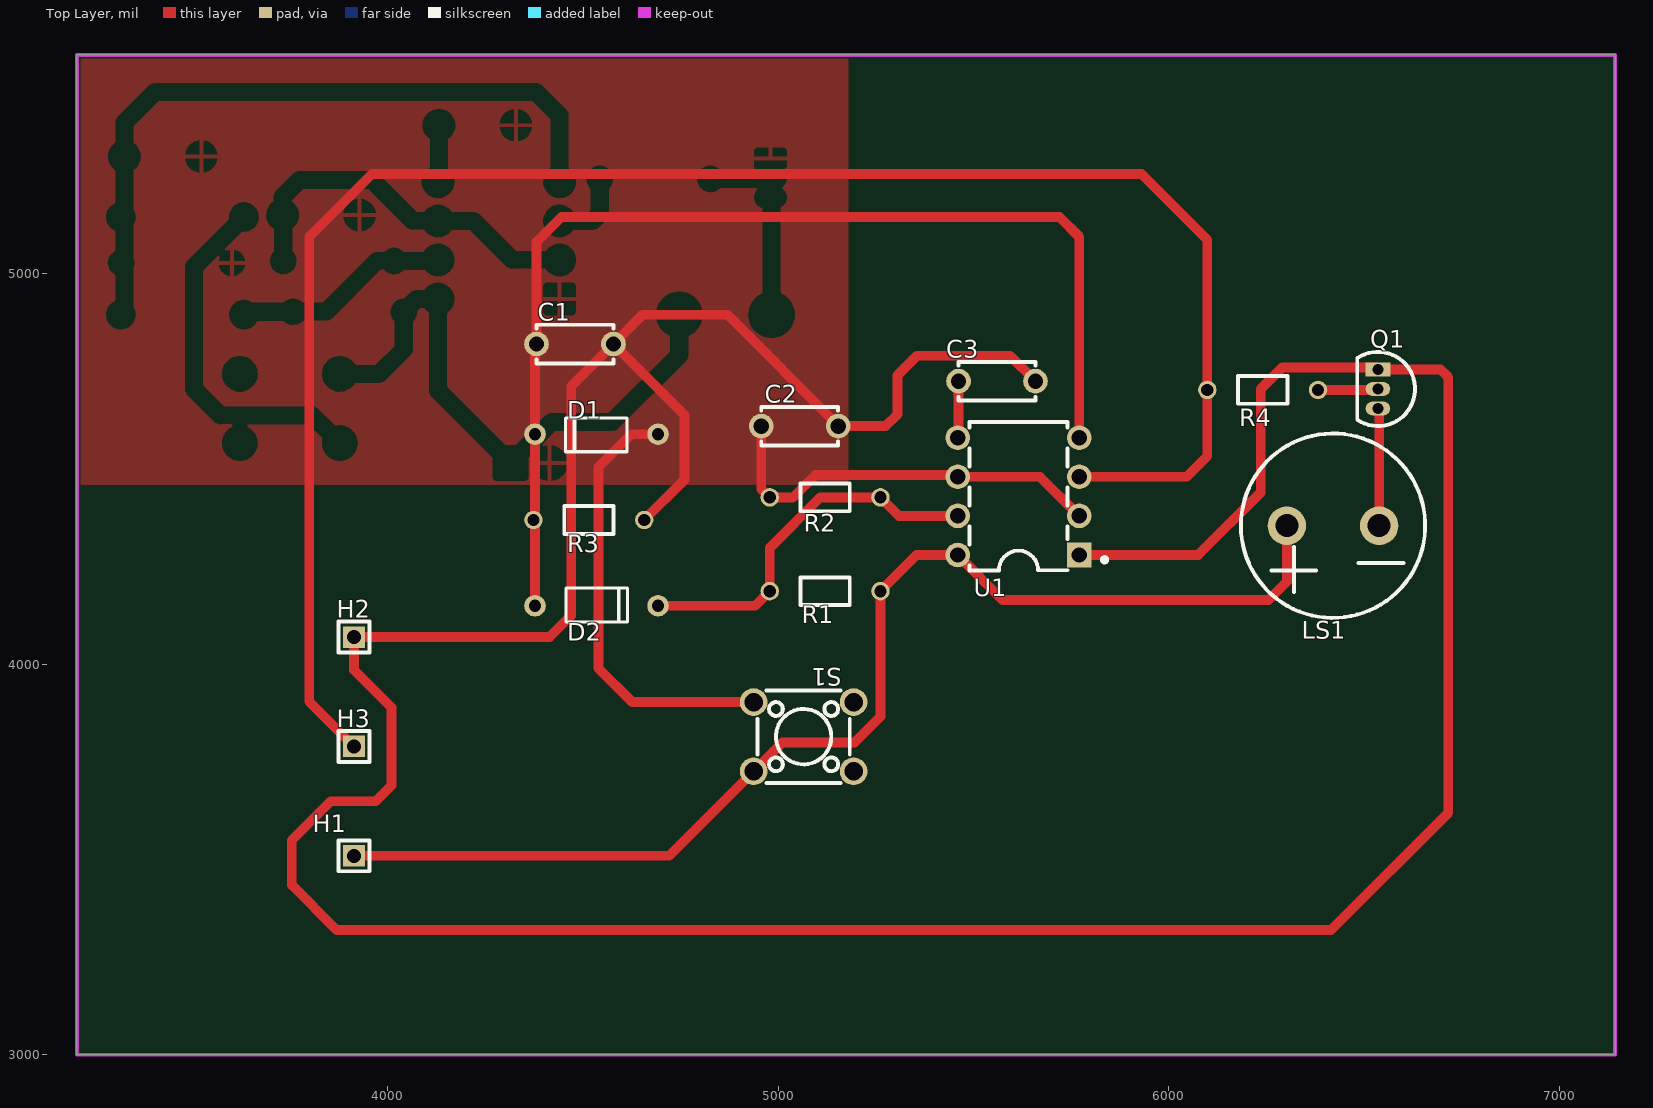
[diagram p0: Top Layer view]
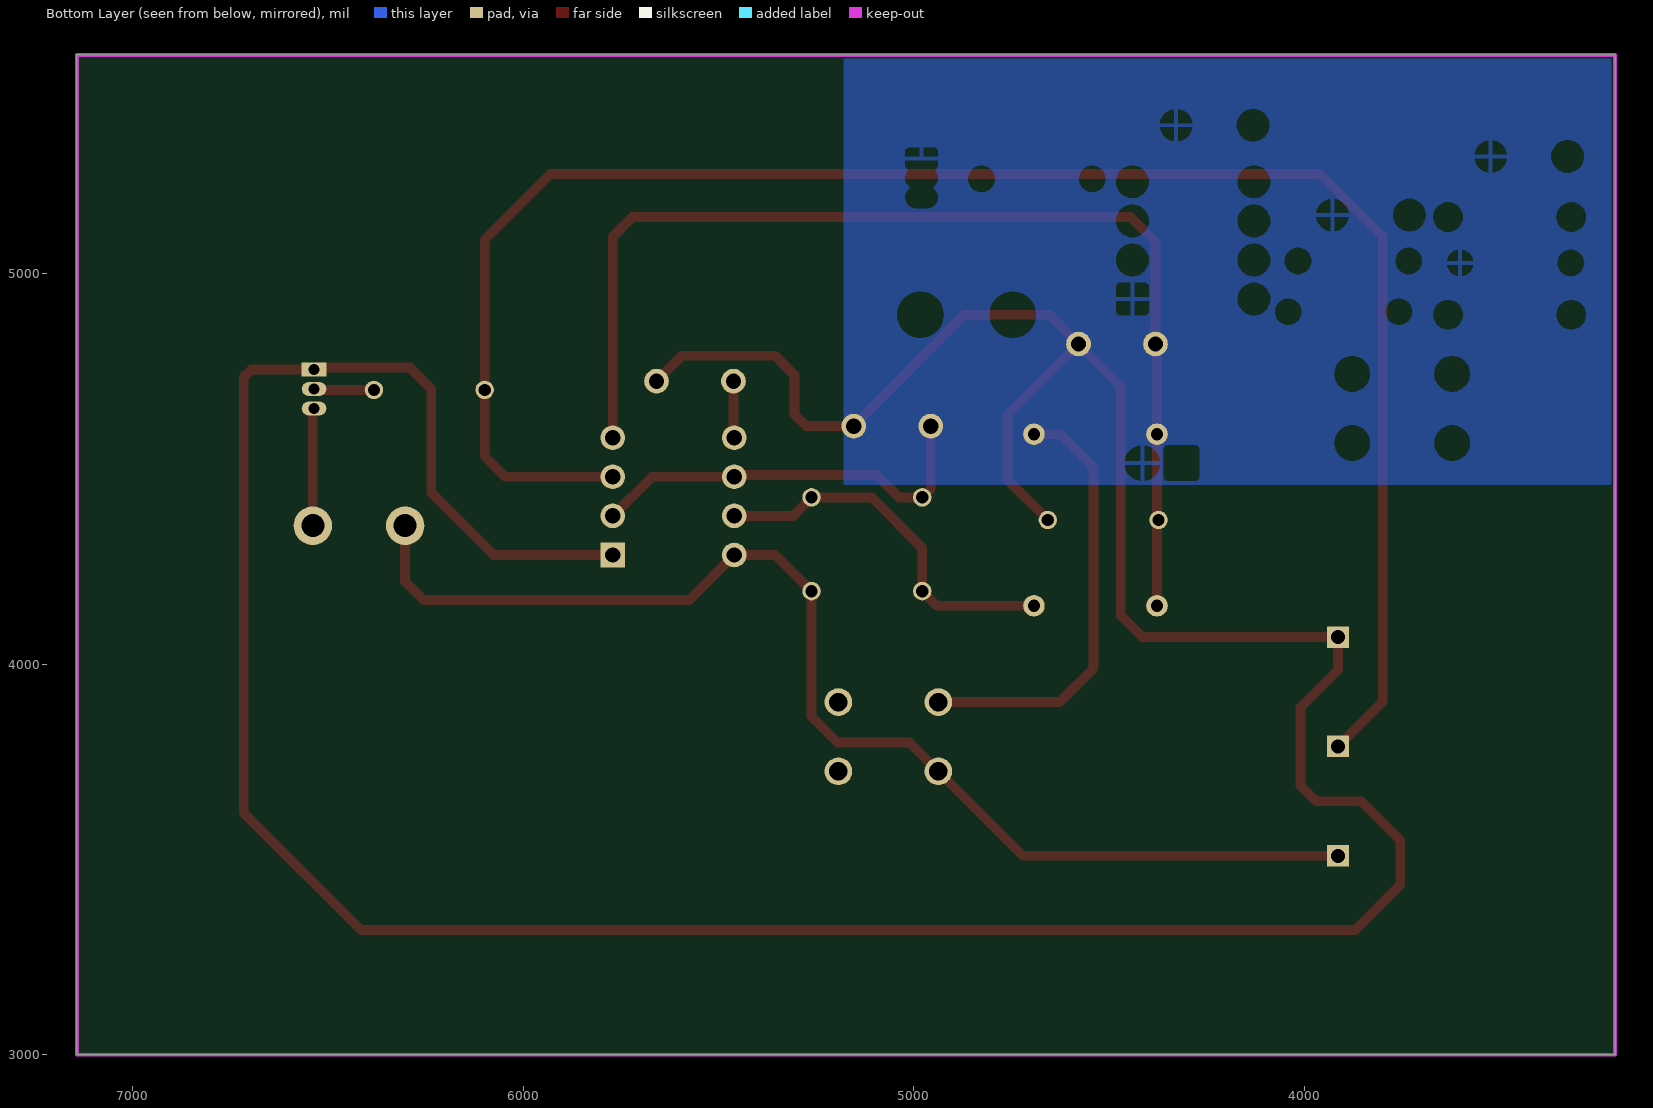
[diagram p1: Bottom Layer view, seen from below]
# Altium PCB MISC52004.pcbdoc
Units mil, origin at the board's own origin, x right, y up, seen from the top; angles counter-clockwise.
Board outline 3937.01 x 2559.06 mil, 2 copper layers (Top Layer, Bottom Layer), stack 62.206 mil thick; 16 components, 10 nets, 38 pads, 0 vias.

## Layer stack, top to bottom
Top Solder Mask Layer: solder mask 0.394, Dk 3.3
Top Layer: signal copper 1.379
Dielectric1: surface 59.449, FR4, Dk 4.5
Bottom Layer: signal copper 1.378
Bottom Solder Mask Layer: solder mask 0.394, Dk 3.3

## Board outline
3205,5559.06 3205,3000 7142.01,3000 7142.01,5559.06

## Design rules (kind name [scope] priority, off if disabled: settings)
BoardOutlineClearance copperThickness2oz_1 [All] p2 off: genericclearance=7.99 ignorepadtopadclearanceinfootprint=FALSE except(0: Arc-SplitContinuation Track-SplitContinuation SMDPad-SplitContinuation THPad-SplitContinuation Via-SplitContinuation Fill-SplitContinuation Region-SplitContinuation Poly-SplitContinuation Text-SplitContinuation Hole-SplitContinuation; 5.98: Arc-CutoutEdge SMDPad-CutoutEdge THPad-CutoutEdge Via-CutoutEdge Fill-CutoutEdge Region-CutoutEdge Text-CutoutEdge; 6.93: Hole-OutlineEdge Hole-CutoutEdge; 10: Poly-OutlineEdge Poly-CutoutEdge; 11.81: Arc-OutlineEdge Track-OutlineEdge SMDPad-OutlineEdge THPad-OutlineEdge Via-OutlineEdge Fill-OutlineEdge Region-OutlineEdge Text-OutlineEdge Track-CutoutEdge)
BoardOutlineClearance copperThickness1oz_1 [All] p4: genericclearance=4.02 ignorepadtopadclearanceinfootprint=FALSE except(0: Arc-SplitContinuation Track-SplitContinuation SMDPad-SplitContinuation THPad-SplitContinuation Via-SplitContinuation Fill-SplitContinuation Region-SplitContinuation Poly-SplitContinuation Text-SplitContinuation Hole-SplitContinuation; 6: SMDPad-CutoutEdge THPad-CutoutEdge Via-CutoutEdge Fill-CutoutEdge Region-CutoutEdge Text-CutoutEdge; 6.93: Hole-OutlineEdge Hole-CutoutEdge; 10: Poly-OutlineEdge Poly-CutoutEdge; 11.8: Arc-OutlineEdge Track-OutlineEdge SMDPad-OutlineEdge THPad-OutlineEdge Via-OutlineEdge Fill-OutlineEdge Region-OutlineEdge Text-OutlineEdge; 11.81: Arc-CutoutEdge Track-CutoutEdge)
Clearance copperThickness2oz [All] p1 off: gap=7.99 ignorepadtopadclearanceinfootprint=FALSE except(5.98: SMDPad-Track SMDPad-SMDPad THPad-Track SMDPad-THPad THPad-THPad Track-Via SMDPad-Via THPad-Via Via-Via Fill-Track Region-Track Fill-SMDPad Region-SMDPad Fill-THPad Region-THPad Fill-Via Region-Via Fill-Fill Fill-Region Region-Region Arc-Track Arc-SMDPad Arc-THPad Arc-Via Fill-Arc Region-Arc Arc-Arc Text-Track SMDPad-Text Text-THPad Text-Via Fill-Text Region-Text Arc-Text Text-Text; 6.93: Hole-Track Hole-SMDPad Hole-THPad Hole-Via Fill-Hole Region-Hole Hole-Arc Hole-Text; 10: Poly-Track Poly-SMDPad Poly-THPad Poly-Via Poly-Fill Poly-Region Poly-Poly Poly-Arc Poly-Text Poly-Hole)
Clearance copperThickness1oz [All] p3: gap=4.02 ignorepadtopadclearanceinfootprint=FALSE except(5.98: SMDPad-Track SMDPad-SMDPad THPad-Track SMDPad-THPad THPad-THPad Track-Via SMDPad-Via THPad-Via Via-Via Fill-Track Region-Track Fill-SMDPad Region-SMDPad Fill-THPad Region-THPad Fill-Via Region-Via Fill-Fill Fill-Region Region-Region; 6: Arc-Track Arc-SMDPad Arc-THPad Arc-Via Fill-Arc Region-Arc Arc-Arc Text-Track SMDPad-Text Text-THPad Text-Via Fill-Text Region-Text Arc-Text Text-Text; 6.93: Hole-Track Hole-SMDPad Hole-THPad Hole-Via Fill-Hole Region-Hole Hole-Arc Hole-Text; 10: Poly-Track Poly-SMDPad Poly-THPad Poly-Via Poly-Fill Poly-Region Poly-Poly Poly-Arc Poly-Text Poly-Hole)
Creepage creepage [All] p1: checkdistance=0 ignoreinternallayers=TRUE applytopolygonpour=TRUE
DiffPairsRouting differentialPair [All] p1: maxlimit=6 minlimit=6 mostfreqgap=6 toplayer_minwidth=5 toplayer_prefwidth=10 toplayer_maxwidth=100 toplayer_mingap=6 toplayer_prefgap=6 toplayer_maxgap=6 bottomlayer_minwidth=5 bottomlayer_prefwidth=10 bottomlayer_maxwidth=100 bottomlayer_mingap=6 bottomlayer_prefgap=6 bottomlayer_maxgap=6 maxuncoupledlength=10
HoleToHoleClearance otherClearance [All] p1: gap=11.81 allowstackedmicrovias=TRUE
Length netLength [All] p1: minlimit=0 maxlimit=0
MatchedLengths netLengthTolerance [All] p1: tolerance=1000
PasteMaskExpansion pasteMaskExpansion [All] p1: expansion=0
PlaneConnect innerPlane [All] p1: planeconnectstyle=Relief reliefexpansion=20 reliefentries=4 reliefconductorwidth=10 reliefairgap=10
PolygonConnect copperRegion [(InNet('GND'))] p1: connectstyle=Relief reliefconductorwidth=10 reliefentries=4 polygonreliefangle="90 Angle" airgapwidth=10 via.connectstyle=Relief via.reliefconductorwidth=10 via.reliefentries=4 via.polygonreliefangle="90 Angle" via.airgapwidth=10
RoutingVias viaSize [All] p1: holewidth=12.01 width=24.02 viastyle="Through Hole" minholewidth=11.81 minwidth=19.68 maxholewidth=248.03 maxwidth=393.7
SolderMaskExpansion solderMaskExpansion [IsVia] p1: expansion=-1000 istentingtop=TRUE
SolderMaskExpansion solderMaskExpansion [All] p2: expansion=2 istentingtop=FALSE
Width copperThickness2oz_2 [All] p1 off: maxlimit=100 minlimit=8 preferedwidth=10
Width copperThickness1oz_2 [All] p2: maxlimit=100 minlimit=5 preferedwidth=10

## Components (designator, comment, footprint, x,y, rotation, side; value= is the part's Value field where it differs from the comment)
C1 "100nF" CAP-TH_L5.0-W2.5-P5.00-D1.0 4479.88,4819.06 r0 top
C2 "0.1uF" CAP-TH_L5.0-W2.5-P5.00-D1.0 5055,4609.06 r0 top
C3 "0.01uF" CAP-TH_L5.0-W2.5-P5.00-D1.0 5560,4724.06 r0 top
D1 "1N4148" DO-35_BD2.2-L4.0-D0.50_1N4148 4535,4588.25 r180 top
D2 "1N4148" DO-35_BD2.2-L4.0-D0.50_1N4148 4535,4149.06 r0 top
H1 "" HDR-TH_1P-V-M_XKB_X4611WV-01I-C28D40 3914.27,3509.06 r0 top
H2 "" HDR-TH_1P-V-M_XKB_X4611WV-01I-C28D40 3914.27,4069.06 r0 top
H3 "" HDR-TH_1P-V-M_XKB_X4611WV-01I-C28D40 3914.27,3789.06 r0 top
LS1 "buzzer" BUZ-TH_BD12.0-P6.00-D0.9-RD 6420,4354.06 r180 top
Q1 "" S8050_TO_92 6535,4704.06 r270 top
R1 "10kΩ" Res_1/8W 5120,4184.06 r0 top
R2 "5kΩ" Res_1/8W 5120,4424.06 r0 top
R3 "10kΩ" Res_1/8W 4515.26,4371.13 r180 top
R4 "120Ω" Res_1/8W 6240,4699.06 r0 top
S1 "" SW-TH_4P-L6.0-W6.0-P4.50-LS6.5 5065,3814.06 r0 top
U1 "LM555CM" PDIP-8_L9.6-W6.4-P2.54-LS7.9-BL-1 5615,4429.06 r90 top

## Footprints (in the part's own frame and the unit in brackets; to place one, negate y for a bottom-side part, rotate by r counter-clockwise, add the part's x,y. Pads: shape width x height; smd on the part's side, far side on the other; paste and mask are expansions set on the pad)
BUZ-TH_BD12.0-P6.00-D0.9-RD [mm]
  round 2.5 hole 1.5 paste+0 mask+0.05: 1(-3,0) 2(3,0)
  silkscreen extent -5.99,-5.99 5.99,5.99
CAP-TH_L5.0-W2.5-P5.00-D1.0 [mm]
  round 1.6 hole 1: 1(-2.5,0) 2(2.5,0)
  silkscreen extent -2.5,-1.27 2.5,1.25
DO-35_BD2.2-L4.0-D0.50_1N4148 [mm]
  round 1.4 hole 0.8 paste+0 mask+0.05: 1(-4,0) 2(4,0)
  silkscreen extent -1.98,-1.06 2.02,1.14
HDR-TH_1P-V-M_XKB_X4611WV-01I-C28D40 [mm]
  rect 1.4x1.4 hole 0.9: 1(0,0)
  silkscreen extent -1,-1 1,1
PDIP-8_L9.6-W6.4-P2.54-LS7.9-BL-1 [mil]
  rect 63x63 hole 39.37: 1(-150,-155.51)
  round 63 hole 39.37: 2(-50,-155.51) 3(50,-155.51) 4(150,-155.51) 5(150,155.52) 6(50,155.52) 7(-50,155.52) 8(-150,155.52)
  silkscreen extent -190,-226 190,125
Res_1/8W [mil]
  round 47.2 hole 31.5 paste+0 mask+2: 1(-141.7,2.48) 2(141.7,2.48)
  silkscreen extent -63,-33 63,38
S8050_TO_92 [mil]
  rect 35.4x63 hole 27.6 paste+0 mask+2: 1(-50,0)
  oval 35.4x63 hole 27.6 paste+0 mask+2: 2(0,0) 3(50,0)
  silkscreen extent -95,-53 95,95
SW-TH_4P-L6.0-W6.0-P4.50-LS6.5 [mm]
  round 1.8 hole 1.2: 1(-3.25,2.25) 2(3.25,2.25) 3(-3.25,-2.25) 4(3.25,-2.25)
  silkscreen extent -3,-3 3,3

## Nets (pads, with @x,y where several pads share a name; then routed paths per layer and width w, separated by ;. In a path a pad name is that pad's centre, name@x,y a point inside that pad or via, vN(x,y) a via of type N, cw(c..) or ccw(c..) an arc to the next point about the centre after c; other vN are vias at no path point)
$1N2: D1.1 S1.1 | length 1135.2
  Top Layer w25: D1.1 4624.19,4588.25 4540,4504.06 4540,3989.06 4626.42,3902.64 S1.1
$1N3: C1.1 D1.2 D2.1 R3.2 U1.4 | length 2883.9
  Top Layer w25: D2.1 D1.2 4377.52,4815.12 C1.1 4381.46,5080.51 4445,5144.06 5720,5144.06 5770.51,5093.55 U1.4
$1N4: D2.2 R1.1 R2.2 U1.7 | length 966.5
  Top Layer w25: D2.2 4940.82,4149.06 R1.1 4978.3,4297.36 5107.48,4426.53 R2.2 5309.18,4379.06 U1.7
$1N7: C2.1 R2.1 U1.2 U1.6 | length 1051.1
  Top Layer w25: C2.1 4956.57,4448.26 R2.1 5037.48,4426.53 5095,4484.06 5454.49,4484.06 U1.6 5670.51,4479.06 U1.2
$1N9: C3.1 U1.5 | length 145.9
  Top Layer w25: U1.5 5461.57,4581.14 C3.1
$1N10: H3.1 R4.1 U1.3 | length 4689.9
  Top Layer w25: H3.1 3800,3903.33 3800,5094.06 3960,5254.06 5930,5254.06 6098.3,5085.76 R4.1 6098.3,4532.36 6045,4479.06 U1.3
$1N11: Q1.2 R4.2 | length 154.3
  Top Layer w25: R4.2 6532.48,4701.53 Q1.2
$1N12: LS1.1 Q1.3 | length 301.3
  Top Layer w25: Q1.3 6538.11,4650.95 LS1.1
GND: C1.2 C2.2 C3.2 H2.1 Q1.1 R3.1 U1.1 | length 9680.4
  Top Layer w25: R3.1 4760,4471.69 4760,4637.36 C1.2 ; C3.2 5593.43,4789.06 5355,4789.06 5305,4739.06 5305,4639.06 5275,4609.06 C2.2 5153.43,4610.63 4870,4894.06 4653.31,4894.06 C1.2 ; U1.1 6075,4279.06 6235,4439.06 6235,4704.06 6290,4759.06 6530,4759.06 Q1.1 6695,4754.06 6715,4734.06 6715,3619.06 6415,3319.06 3870,3319.06 3755,3434.06 3755,3549.06 3855,3649.06 3970,3649.06 4010,3689.06 4010,3889.06 3914.27,3984.79 H2.1 4415,4069.06 4470,4124.06 4470,4710.75 C1.2
VCC: H1.1 LS1.2 R1.2 S1.3 U1.8 | length 3104.6
  Top Layer w25: H1.1 4720.63,3509.06 S1.3 5010.63,3799.06 5195,3799.06 5261.7,3865.76 R1.2 5354.22,4279.06 U1.8 5574.49,4164.06 6255,4164.06 6301.89,4210.95 LS1.2
pads on no net: S1.2 S1.4

## Polygon pours and split planes (outlines as drawn)
GND on Top Layer (solid, remove dead copper, pour order 0): 3000,5679.06 3000,4259.06 5570,4259.06 5570,5679.06
GND on Bottom Layer (solid, remove dead copper, pour order 2): 3105,5679.06 3105,4374.06 5370,4374.06 5370,5679.06

## Keep-outs
Board Outline Layer:
  the board outline again, w10

## Dimensions
3205,5559.06 to 7142.01,5559.06 on Document Layer
7235,3000 to 7235,5559.06 on Document Layer